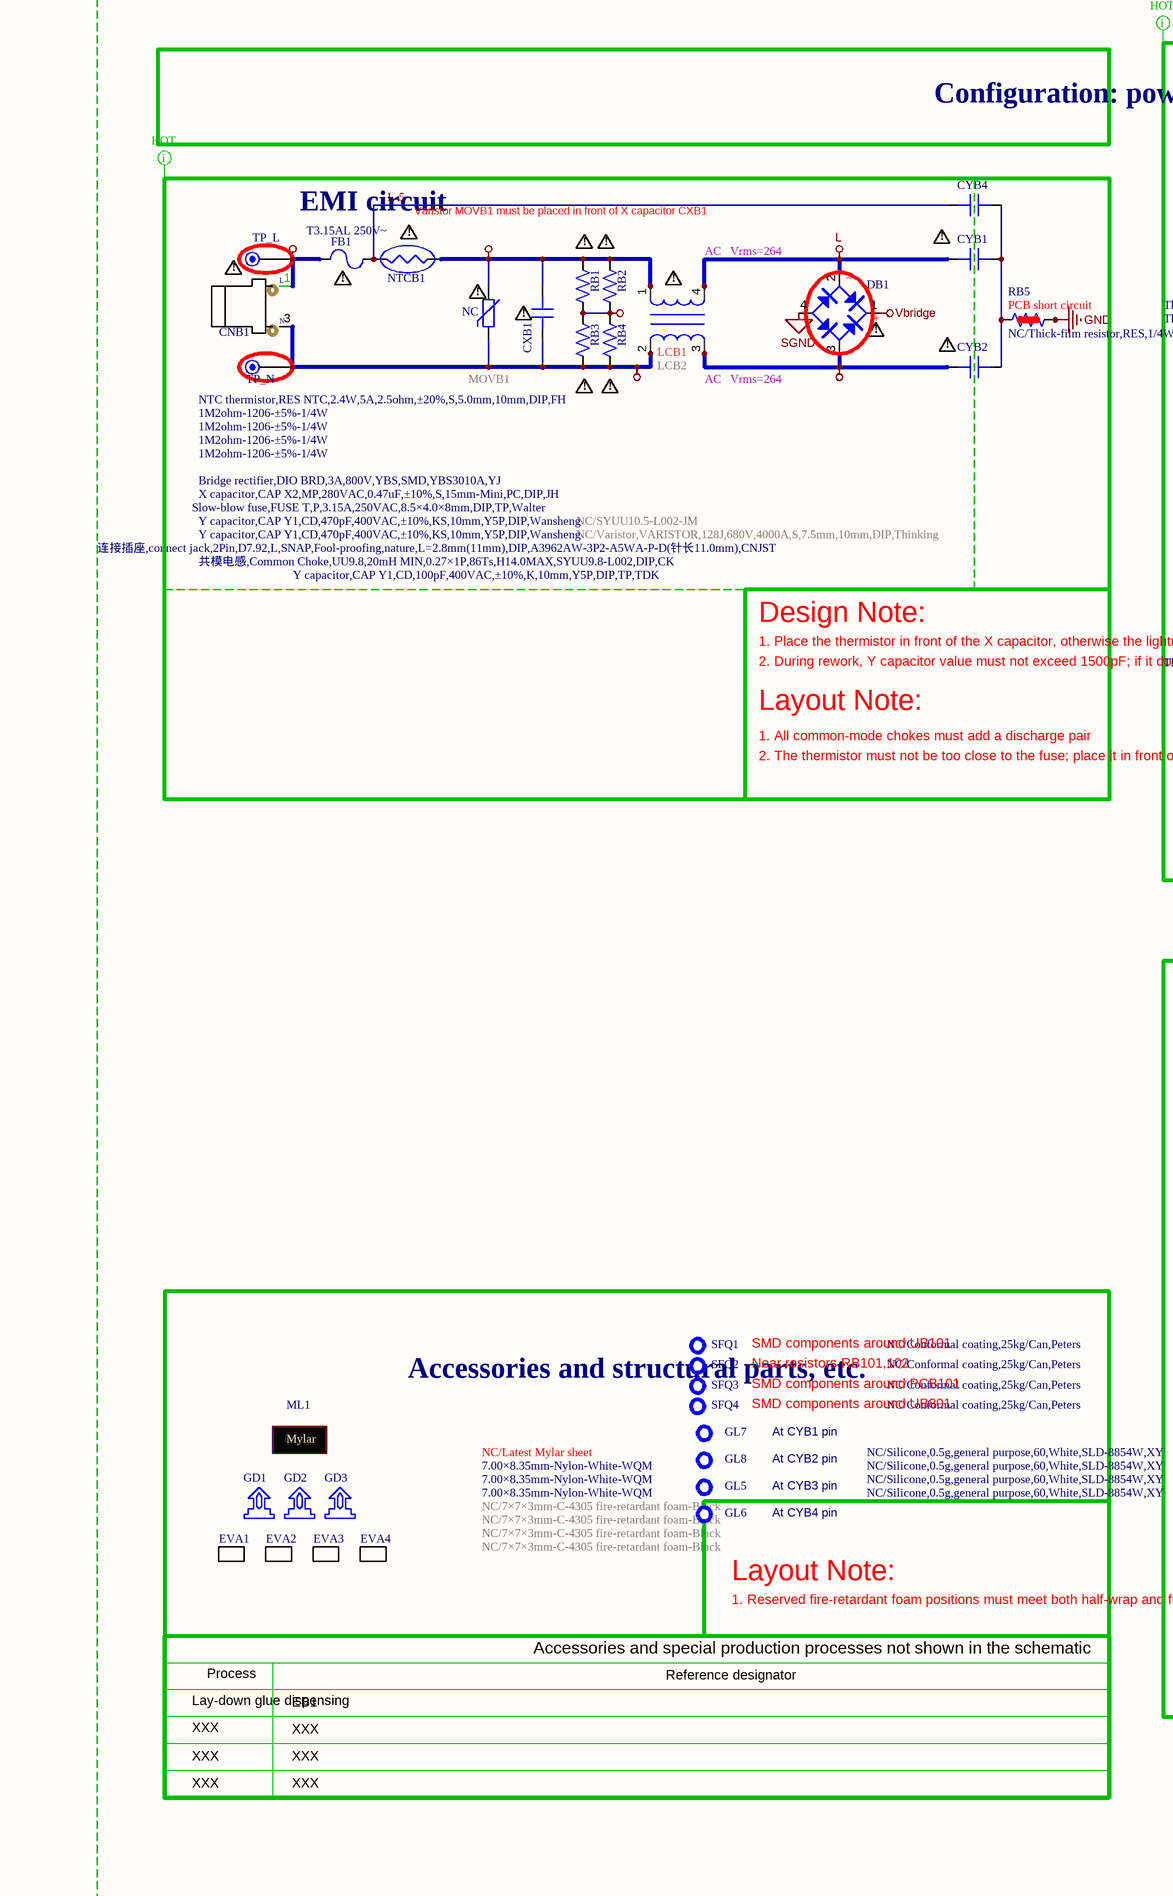
[diagram p0: MISC116569-4.SchDoc, left]
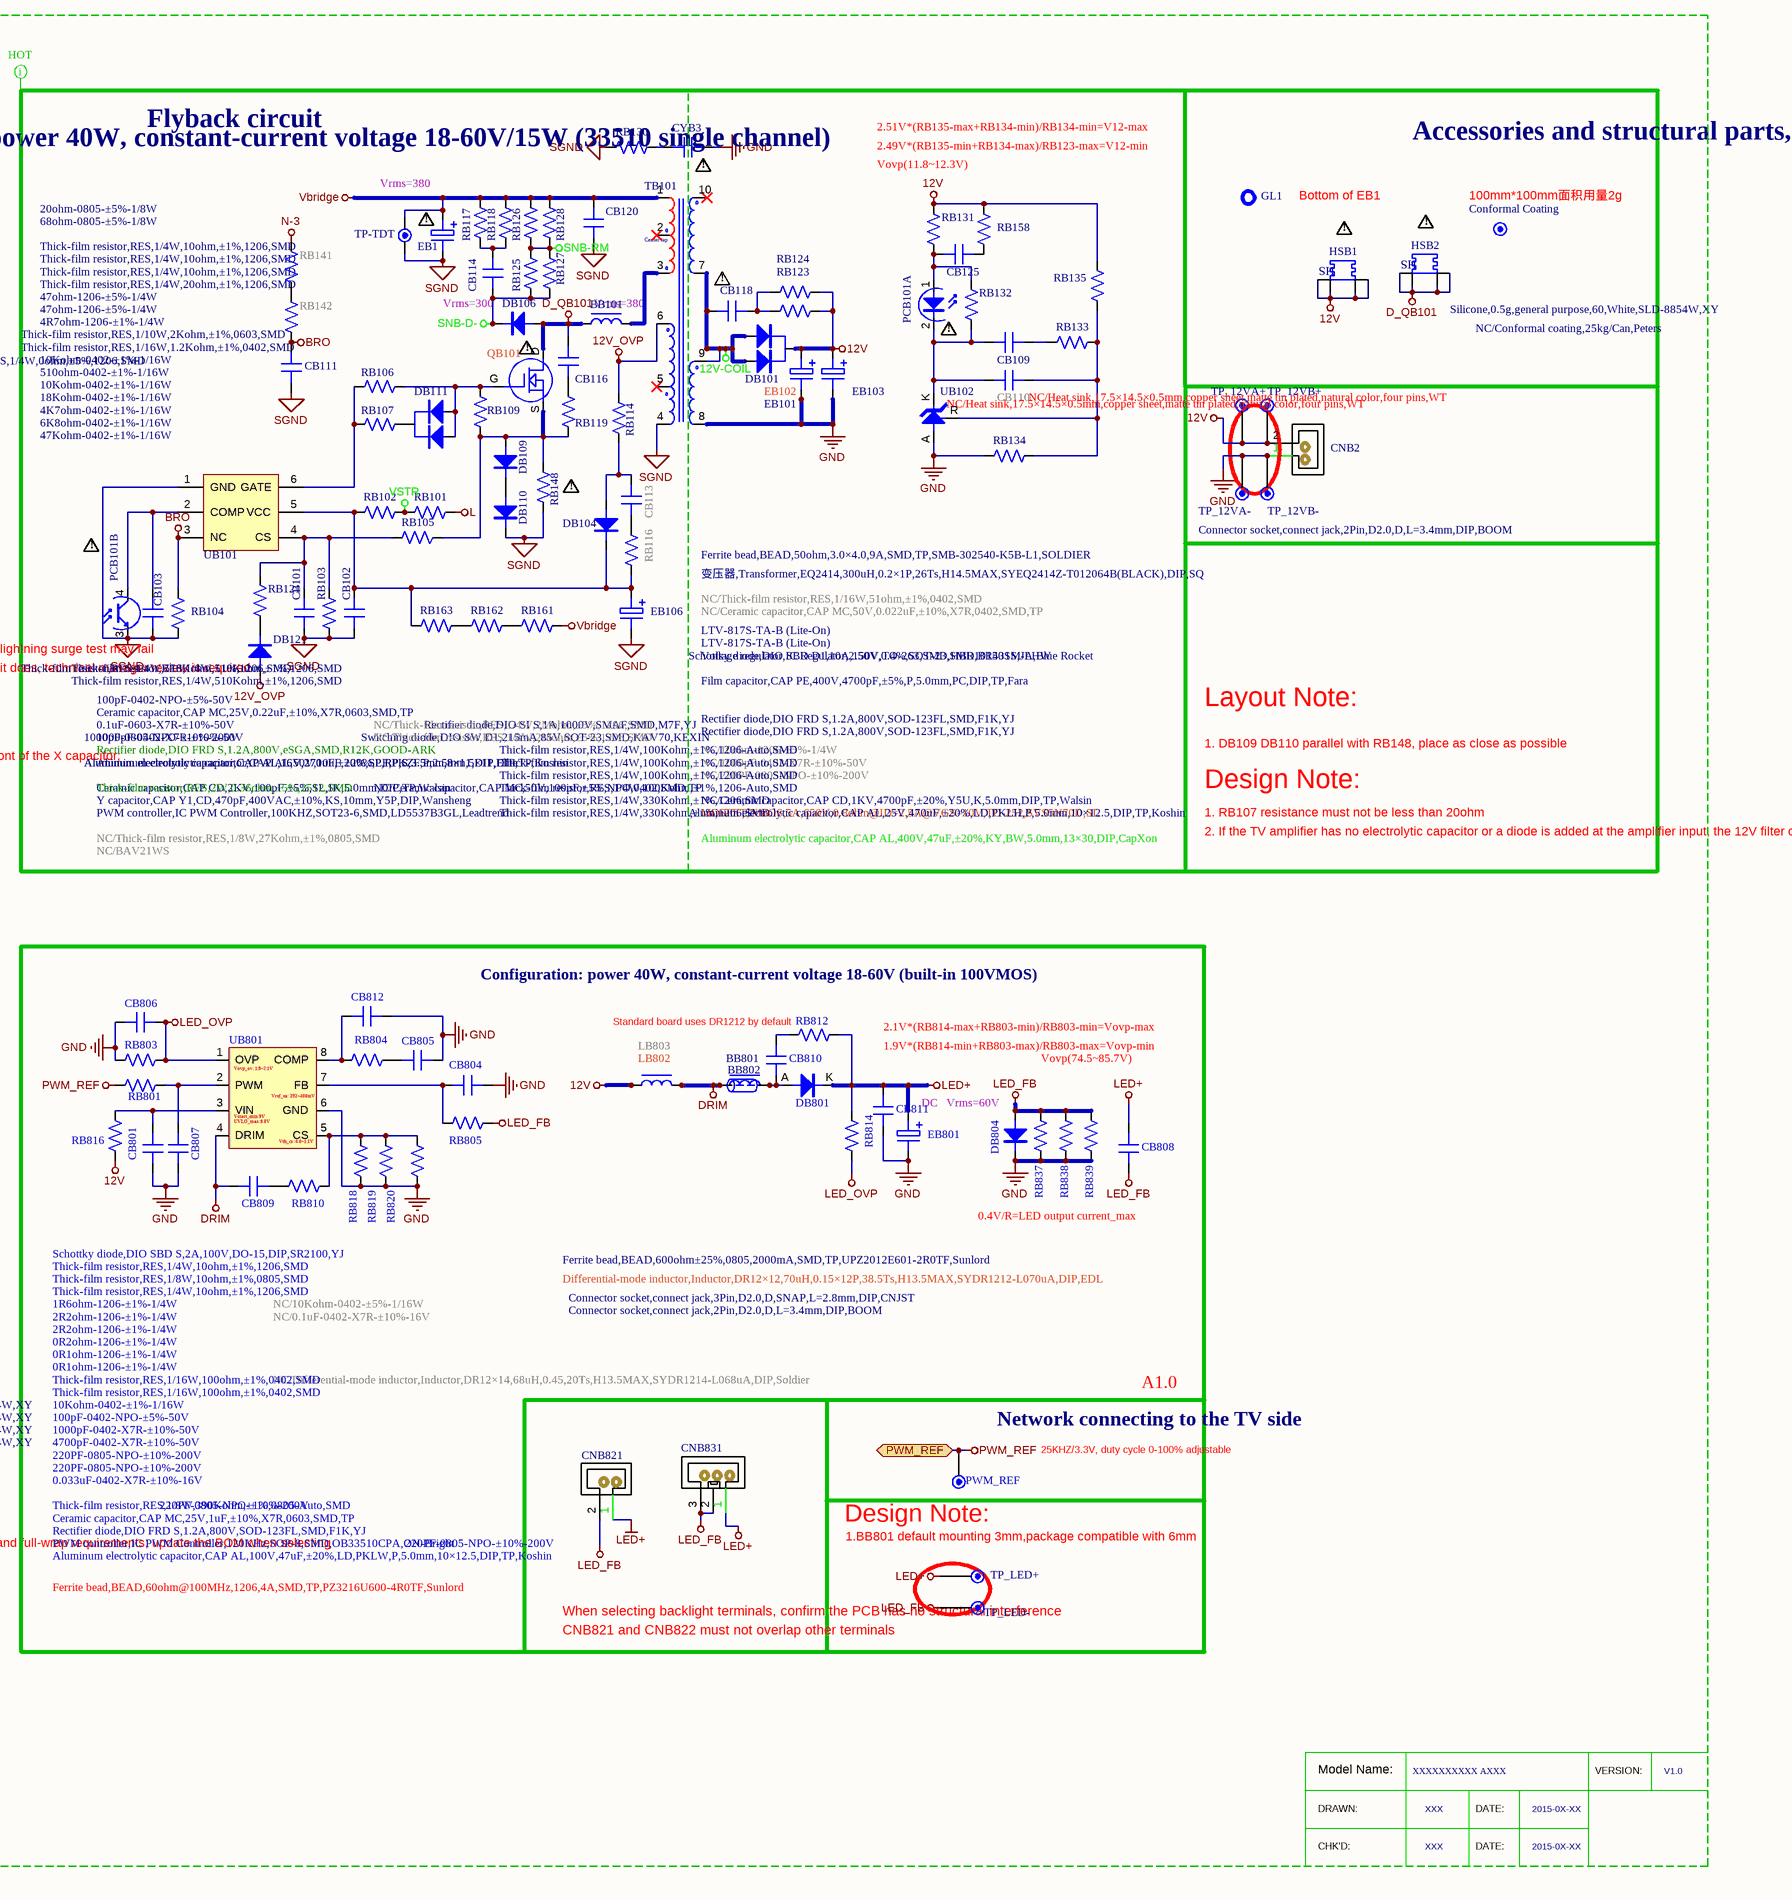
[diagram p1: MISC116569-4.SchDoc, right]
# Altium project MISC116569-15.PrjPCB (part 7 of 8)

## Sheet MISC116569-4.SchDoc: MISC116569
size A2

### Parts
BB101  Ferrite bead,BEAD,50ohm,3.0×4.0,9A,SMD,TP,SMB-302540-K5B-L1,SOLDIER  [L(4*3*2.55)-S]
BB801  Ferrite bead,BEAD,60ohm@100MHz,1206,4A,SMD,TP,PZ3216U600-4R0TF,Sunlord  [L1206]
BB802  Ferrite bead,BEAD,600ohm±25%,0805,2000mA,SMD,TP,UPZ2012E601-2R0TF,Sunlord  [L0805]
CB101  100pF-0402-NPO-±5%-50V  [C0402]
CB102  0.1uF-0603-X7R-±10%-50V  [C0603]
CB103  1000pF-0402-X7R-±10%-50V  [C0402]
CB109  Ceramic capacitor,CAP MC,25V,0.22uF,±10%,X7R,0603,SMD,TP  [C0603]
CB110  NC/1000pF-0402-X7R-±10%-50V  [C0402]
CB111  NC/Ceramic capacitor,CAP MC,50V,100pF,±5%,NPO,0402,SMD,TP  [C0402]
CB113  NC/220PF-0805-NPO-±10%-200V  [C0805]
CB114  Film capacitor,CAP PE,400V,4700pF,±5%,P,5.0mm,PC,DIP,TP,Fara  [CAP8*2.5-V-5]
CB116  Ceramic capacitor,CAP CD,2KV,100pF,±5%,SL,IK,5.0mm,DIP,TP,Walsin  [CAP6.5*5-V-5-1]
CB118  1000pF-0805-NPO-±10%-200V  [C0805]
CB120  NC/Ceramic capacitor,CAP CD,1KV,4700pF,±20%,Y5U,K,5.0mm,DIP,TP,Walsin  [CAP10*4.5-V-5]
CB125  NC/Ceramic capacitor,CAP MC,50V,0.022uF,±10%,X7R,0402,SMD,TP  [C0402]
CB801  Ceramic capacitor,CAP MC,25V,1uF,±10%,X7R,0603,SMD,TP  [C0603]
CB804  4700pF-0402-X7R-±10%-50V  [C0402]
CB805  NC/0.1uF-0402-X7R-±10%-16V  [C0402]
CB806  1000pF-0402-X7R-±10%-50V  [C0402]
CB807  100pF-0402-NPO-±5%-50V  [C0402]
CB808  220PF-0805-NPO-±10%-200V  [C0805]
CB809  220PF-0805-NPO-±10%-200V  [C0805]
CB810  220PF-0805-NPO-±10%-200V  [C0805]
CB811  220PF-0805-NPO-±10%-200V  [C0805]
CB812  0.033uF-0402-X7R-±10%-16V  [C0402]
CNB1  连接插座,connect jack,2Pin,D7.92,L,SNAP,Fool-proofing,nature,L=2.8mm(11mm),DIP,A3962AW-3P2-A5WA-P-D(针长11.0mm),CNJST  [CON2-H7.92]
CNB2  Connector socket,connect jack,2Pin,D2.0,D,L=3.4mm,DIP,BOOM  [SIP2/2.0D-1]
CNB821  Connector socket,connect jack,2Pin,D2.0,D,L=3.4mm,DIP,BOOM  [SIP2/2.0D-1]
CNB831  Connector socket,connect jack,3Pin,D2.0,D,SNAP,L=2.8mm,DIP,CNJST  [SIP3/2.0D-3]
Conformal_Coating  NC/Conformal coating,25kg/Can,Peters  [Conformal Coating]
CXB1  X capacitor,CAP X2,MP,280VAC,0.47uF,±10%,S,15mm-Mini,PC,DIP,JH  [CAP18*8.5-V-15]
CYB1  Y capacitor,CAP Y1,CD,470pF,400VAC,±10%,KS,10mm,Y5P,DIP,Wansheng  [CAP13*5-V-10-1]
CYB2  Y capacitor,CAP Y1,CD,470pF,400VAC,±10%,KS,10mm,Y5P,DIP,Wansheng  [CAP13*5-V-10-1]
CYB3  Y capacitor,CAP Y1,CD,470pF,400VAC,±10%,KS,10mm,Y5P,DIP,Wansheng  [CAP13*5-V-10-1]
CYB4  Y capacitor,CAP Y1,CD,100pF,400VAC,±10%,K,10mm,Y5P,DIP,TP,TDK  [CAP13*5-V-10-1]
DB1  Bridge rectifier,DIO BRD,3A,800V,YBS,SMD,YBS3010A,YJ  [B/YBS3010A]
DB101  Schottky diode,DIO SBD D1,10A,150V,TO-263,SMD,HBR10150SS,JLHW  [D2PAK3]
DB104  Rectifier diode,DIO SI S,1A,1000V,SMAF,SMD,M7F,YJ  [DIODE-S-1]
DB106  Rectifier diode,DIO FRD S,1.2A,800V,eSGA,SMD,R12K,GOOD-ARK  [DIODE-S-14]
DB109  Rectifier diode,DIO FRD S,1.2A,800V,SOD-123FL,SMD,F1K,YJ  [DIODE-S-14]
DB110  Rectifier diode,DIO FRD S,1.2A,800V,SOD-123FL,SMD,F1K,YJ  [DIODE-S-14]
DB111  Switching diode,DIO SW D1,215mA,85V,SOT-23,SMD,KAV70,KEXIN  [SO-23]
DB121  NC/BAV21WS  [DIODE-S-12]
DB801  Schottky diode,DIO SBD S,2A,100V,DO-15,DIP,SR2100,YJ  [D2-H-15]
DB804  Rectifier diode,DIO FRD S,1.2A,800V,SOD-123FL,SMD,F1K,YJ  [DIODE-S-14]
EB1  Aluminum electrolytic capacitor,CAP AL,400V,47uF,±20%,KY,BW,5.0mm,13×30,DIP,CapXon  [EC(13*30)-H-5]
EB101  Aluminum electrolytic capacitor,CAP AL,16V,270uF,±20%,SP,RP,S,3.5mm,8×11,DIP,Elite  [EC(8*11)-V-3.5]
EB102  Aluminum electrolytic capacitor,CAP AL,25V,470uF,±20%,LD,PKLH,P,5.0mm,10×12.5,DIP,TP,Koshin  [EC(10*12.5)-V-5]
EB103  Aluminum electrolytic capacitor,CAP AL,16V,270uF,±20%,SP,RP,S,3.5mm,8×11,DIP,Elite  [EC(8*11)-V-3.5]
EB106  Aluminum electrolytic capacitor,CAP AL,50V,10uF,±20%,LF,PKZF,P,2.5mm,5×11,DIP,TP,Koshin  [EC(5*11)-V-2.5]
EB801  Aluminum electrolytic capacitor,CAP AL,100V,47uF,±20%,LD,PKLW,P,5.0mm,10×12.5,DIP,TP,Koshin  [EC(10*12.5)-V-5]
EVA1  NC/7×7×3mm-C-4305 fire-retardant foam-Black  [EVA(7*7*3)]
EVA2  NC/7×7×3mm-C-4305 fire-retardant foam-Black  [EVA(7*7*3)]
EVA3  NC/7×7×3mm-C-4305 fire-retardant foam-Black  [EVA(7*7*3)]
EVA4  NC/7×7×3mm-C-4305 fire-retardant foam-Black  [EVA(7*7*3)]
FB1  Slow-blow fuse,FUSE T,P,3.15A,250VAC,8.5×4.0×8mm,DIP,TP,Walter  [FUSE8.5*4-V-5(T3.15AL 250V~)]
GD1  7.00×8.35mm-Nylon-White-WQM  [Fixed]
GD2  7.00×8.35mm-Nylon-White-WQM  [Fixed]
GD3  7.00×8.35mm-Nylon-White-WQM  [Fixed]
GL1  Silicone,0.5g,general purpose,60,White,SLD-8854W,XY  [Silica gel-15]
GL5  NC/Silicone,0.5g,general purpose,60,White,SLD-8854W,XY  [Silica gel-10]
GL6  NC/Silicone,0.5g,general purpose,60,White,SLD-8854W,XY  [Silica gel-10]
GL7  NC/Silicone,0.5g,general purpose,60,White,SLD-8854W,XY  [Silica gel-10]
GL8  NC/Silicone,0.5g,general purpose,60,White,SLD-8854W,XY  [Silica gel-10]
HSB1  NC/Heat sink,17.5×14.5×0.5mm,copper sheet,matte tin plated,natural color,four pins,WT  [HS151-TEMP-NG]
HSB2  NC/Heat sink,17.5×14.5×0.5mm,copper sheet,matte tin plated,natural color,four pins,WT  [HS151-TEMP-NG]
LB802  Differential-mode inductor,Inductor,DR12×12,70uH,0.15×12P,38.5Ts,H13.5MAX,SYDR1212-L070uA,DIP,EDL  [L/LC2/15*14.5-V7.5]
LB803  NC/Differential-mode inductor,Inductor,DR12×14,68uH,0.45,20Ts,H13.5MAX,SYDR1214-L068uA,DIP,Soldier  [L(13.5*15.5)-V-5]
LCB1  共模电感,Common Choke,UU9.8,20mH MIN,0.27×1P,86Ts,H14.0MAX,SYUU9.8-L002,DIP,CK  [L/LC4/UU9.8/7*8-H]
LCB2  NC/SYUU10.5-L002-JM  [L/UU10.5/10*13-2]
ML1  NC/Latest Mylar sheet  [Mylar]
MOVB1  NC/Varistor,VARISTOR,128J,680V,4000A,S,7.5mm,10mm,DIP,Thinking  [VR(13*5)-V-7.5]
NTCB1  NTC thermistor,RES NTC,2.4W,5A,2.5ohm,±20%,S,5.0mm,10mm,DIP,FH  [NTC(10*5)-V5]
PCB101  LTV-817S-TA-B (Lite-On)  [OC4-S-1]  (parts A,B of 2)
PWM_REF  NC/TEST  [TP_BL]  (value not drawn)
QB101  MOSFET,NMOS,5A,650V,0.8ohm@ID=2.5A@VGS=10V,TO-252,SVS5N70D,SL  [TO-252-GDS]
RB1  1M2ohm-1206-±5%-1/4W  [R1206]
RB2  1M2ohm-1206-±5%-1/4W  [R1206]
RB3  1M2ohm-1206-±5%-1/4W  [R1206]
RB4  1M2ohm-1206-±5%-1/4W  [R1206]
RB5  NC/Thick-film resistor,RES,1/4W,0ohm,±5%,1206,SMD  [R1206SC]
RB101  Thick-film resistor,RES,1/4W,330Kohm,±1%,1206,SMD  [R1206]
RB102  Thick-film resistor,RES,1/4W,330Kohm,±1%,1206,SMD  [R1206]
RB103  6K8ohm-0402-±1%-1/16W  [R0402]
RB104  47Kohm-0402-±1%-1/16W  [R0402]
RB105  510ohm-0402-±1%-1/16W  [R0402]
RB106  68ohm-0805-±5%-1/8W  [R0805]
RB107  20ohm-0805-±5%-1/8W  [R0805]
RB109  10Kohm-0402-±1%-1/16W  [R0402]
RB114  4R7ohm-1206-±1%-1/4W  [R1206]
RB116  NC/10ohm-1206-±5%-1/4W  [R1206]
RB117  Thick-film resistor,RES,1/4W,10ohm,±1%,1206,SMD  [R1206]
RB118  Thick-film resistor,RES,1/4W,10ohm,±1%,1206,SMD  [R1206]
RB119  Thick-film resistor,RES,1/4W,10ohm,±1%,1206,SMD  [R1206]
RB121  NC/Thick-film resistor,RES,1/8W,27Kohm,±1%,0805,SMD  [R0805]
RB123  47ohm-1206-±5%-1/4W  [R1206]
RB124  47ohm-1206-±5%-1/4W  [R1206]
RB125  Thick-film resistor,RES,1/4W,100Kohm,±1%,1206-Auto,SMD  [R1206]
RB126  Thick-film resistor,RES,1/4W,100Kohm,±1%,1206-Auto,SMD  [R1206]
RB127  Thick-film resistor,RES,1/4W,100Kohm,±1%,1206-Auto,SMD  [R1206]
RB128  Thick-film resistor,RES,1/4W,100Kohm,±1%,1206-Auto,SMD  [R1206]
RB130  Thick-film resistor,RES,1/4W,20ohm,±1%,1206,SMD  [R1206]
RB131  Thick-film resistor,RES,1/10W,2Kohm,±1%,0603,SMD  [R0603]
RB132  Thick-film resistor,RES,1/16W,1.2Kohm,±1%,0402,SMD  [R0402]
RB133  10Kohm-0402-±1%-1/16W  [R0402]
RB134  4K7ohm-0402-±1%-1/16W  [R0402]
RB135  18Kohm-0402-±1%-1/16W  [R0402]
RB141  NC/Thick-film resistor,RES,1/4W,2Mohm,±5%,1206,SMD  [R1206]
RB142  NC/Thick-film resistor,RES,1/4W,2Mohm,±5%,1206,SMD  [R1206]
RB148  Thick-film resistor,RES,2W,0.36ohm,±5%,2512,SMD  [R2512-1]
RB158  NC/Thick-film resistor,RES,1/16W,51ohm,±1%,0402,SMD  [R0402]
RB161  Thick-film resistor,RES,1/4W,510Kohm,±1%,1206,SMD  [R1206]
RB162  Thick-film resistor,RES,1/4W,510Kohm,±1%,1206,SMD  [R1206]
RB163  Thick-film resistor,RES,1/4W,510Kohm,±1%,1206,SMD  [R1206]
RB801  Thick-film resistor,RES,1/16W,100ohm,±1%,0402,SMD  [R0402]
RB803  10Kohm-0402-±1%-1/16W  [R0402]
RB804  NC/10Kohm-0402-±5%-1/16W  [R0402]
RB805  Thick-film resistor,RES,1/16W,100ohm,±1%,0402,SMD  [R0402]
RB810  Thick-film resistor,RES,1/4W,10ohm,±1%,1206,SMD  [R1206]
RB812  Thick-film resistor,RES,1/4W,10ohm,±1%,1206,SMD  [R1206]
RB814  Thick-film resistor,RES,1/8W,390Kohm,±1%,0805-Auto,SMD  [R0805]
RB816  Thick-film resistor,RES,1/8W,10ohm,±1%,0805,SMD  [R0805]
RB818  0R2ohm-1206-±1%-1/4W  [R1206]
RB819  0R1ohm-1206-±1%-1/4W  [R1206]
RB820  0R1ohm-1206-±1%-1/4W  [R1206]
RB837  1R6ohm-1206-±1%-1/4W  [R1206]
RB838  2R2ohm-1206-±1%-1/4W  [R1206]
RB839  2R2ohm-1206-±1%-1/4W  [R1206]
SFQ1  NC/Conformal coating,25kg/Can,Peters  [SFQ]
SFQ2  NC/Conformal coating,25kg/Can,Peters  [SFQ]
SFQ3  NC/Conformal coating,25kg/Can,Peters  [SFQ]
SFQ4  NC/Conformal coating,25kg/Can,Peters  [SFQ]
TB101  变压器,Transformer,EQ2414,300uH,0.2×1P,26Ts,H14.5MAX,SYEQ2414Z-T012064B(BLACK),DIP,SQ  [T/EQ2414*10]
TP-TDT  NC/  [TP-TDT]  (value not drawn)
TP_12VA+  NC/  [TP]  (value not drawn)
TP_12VA-  NC/  [TP]  (value not drawn)
TP_12VB+  NC/  [TP]  (value not drawn)
TP_12VB-  NC/  [TP]  (value not drawn)
TP_L  NC/  [TP-80]  (value not drawn)
TP_LED+  NC/  [TP]  (value not drawn)
TP_LED-  NC/  [TP]  (value not drawn)
TP_N  NC/  [TP-80]  (value not drawn)
UB101  PWM controller,IC PWM Controller,100KHZ,SOT23-6,SMD,LD5537B3GL,Leadtrend  [SOT-26]
UB102  Voltage regulator,IC Regulator,2.50V,0.4%,SOT-23,SMD,BR431M-A,Blue Rocket  [SOT-23-RAK]
UB801  PWM controller,IC PWM Controller,120KHz,SOP-8,SMD,OB33510CPA,ON-Bright  [SO-8A]

### Blocks framed on the sheet
Design Note:: BB801 BB802 CB801 CB804-CB812 CNB821 CNB831 DB801 DB804 EB801 LB802 LB803 PWM_REF RB801 RB803-RB805 RB810 RB812 RB814 RB816 RB818-RB820 RB837-RB839 TP_LED+ TP_LED- UB801

### Ports
PWM_REF

### Nets
12V: CNB2.2 DB101.2 EB101.1 EB102.1 EB103.1 HSB1.1 HSB1.2 HSB1.3 HSB1.4 LB802.1 LB803.1 RB123.2 RB124.2 RB131.2 RB135.1 RB158.2 RB816.1 TP_12VA+.1 TP_12VB+.1
12V-COIL: CB118.1 DB101.1 DB101.3 TB101.7 TB101.9
12V_OVP: DB121.A RB114.2 TB101.6
BRO: CB111.1 RB104.1 RB142.1 UB101.3(NC)
D_QB101: BB101.1 CB116.2 DB106.A HSB2.1 HSB2.2 HSB2.3 HSB2.4 QB101.D
DRIM: BB801.1 BB802.1 CB809.2 LB802.2 LB803.2 UB801.4(DRIM)
GND: CB801.2 CB804.1 CB805.2 CB806.2 CB807.1 CB811.1 CB812.2 CNB2.1 CYB3.2 DB804.K EB101.2 EB102.2 EB103.2 EB801.2 RB5.2 RB5.3 RB134.1 RB803.1 RB818.1 RB819.1 RB820.1 RB837.1 RB838.1 RB839.2 TB101.8 TP_12VA-.1 TP_12VB-.1 UB102.A UB801.6(GND)
L: CYB1.1 DB1.2 LCB1.4 LCB2.4 RB101.1
L-1: CNB1.1 FB1.1 TP_L.1
L-2: CXB1.1 LCB1.1 LCB2.1 MOVB1.1 NTCB1.1 RB1.1 RB2.1
L-N: RB1.2 RB2.2 RB3.1 RB4.1
LED+: CB808.2 CB811.2 CNB821.1 CNB831.1 DB801.K EB801.1 RB812.2 RB814.2 TP_LED+.1
LED_FB: CB808.1 CNB821.2 CNB831.2 CNB831.3 DB804.A RB805.2 RB837.2 RB838.2 RB839.1 TP_LED-.1
LED_OVP: CB806.1 RB803.2 RB814.1 UB801.1(OVP)
N-2: CNB1.3 CXB1.2 LCB1.2 LCB2.2 MOVB1.2 RB3.2 RB4.2 TP_N.1
N-3: CYB2.1 DB1.3 LCB1.3 LCB2.3 RB141.2
PWM_REF: PWM_REF.1 RB801.1 ; port PWM_REF
SGND: CB101.2 CB102.2 CB103.1 CB111.2 CB120.1 DB1.4 DB110.K EB1.2 EB106.2 PCB101.3 RB103.1 RB104.2 RB130.1 RB148.1 TB101.4 TP-TDT.2 UB101.1(GND)
SNB-D-: CB114.2 DB106.K RB125.1 RB127.1
SNB-RM: RB125.2 RB126.1 RB127.2 RB128.1
Vbridge: CB120.2 DB1.1 EB1.1 RB117.2 RB118.2 RB126.2 RB128.2 RB161.1 TB101.1 TP-TDT.1
VSTR: RB101.2 RB102.1
L-5: CYB4.1 FB1.2 NTCB1.2
NetBB101_2: BB101.2 TB101.3
NetBB801_2: BB801.2 BB802.2 CB810.1 DB801.A
NetCB101_1: CB101.1 RB103.2 RB105.1 RB121.2 UB101.4(CS)
NetCB102_1: CB102.1 DB104.K EB106.1 RB102.2 RB116.1 RB163.2 UB101.5(VCC)
NetCB103_2: CB103.2 PCB101.4 UB101.2(COMP)
NetCB109_1: CB109.1 CB110.1 PCB101.2 RB132.1 UB102.K
NetCB109_2: CB109.2 RB133.1
NetCB110_2: CB110.2 RB133.2 RB134.2 RB135.2 UB102.R
NetCB113_1: CB113.1 DB104.A RB114.1
NetCB113_2: CB113.2 RB116.2
NetCB114_1: CB114.1 RB117.1 RB118.1
NetCB116_1: CB116.1 RB119.2
NetCB118_2: CB118.2 RB123.1 RB124.1
NetCB125_1: CB125.1 PCB101.1 RB131.1 RB132.2
NetCB125_2: CB125.2 RB158.1
NetCB801_1: CB801.1 RB816.2 UB801.3(VIN)
NetCB804_2: CB804.2 RB805.1 UB801.7(FB)
NetCB805_1: CB805.1 RB804.2
NetCB807_2: CB807.2 RB801.2 UB801.2(PWM)
NetCB809_1: CB809.1 RB810.2
NetCB810_2: CB810.2 RB812.1
NetCB812_1: CB812.1 RB804.1 UB801.8(COMP)
NetCYB1_2: CYB1.2 CYB2.2 CYB4.2 RB5.1
NetCYB3_1: CYB3.1 RB130.2
NetDB109_A: DB109.A QB101.S RB105.2 RB109.2 RB119.1 RB148.2
NetDB109_K: DB109.K DB110.A
NetDB111_1: DB111.1 DB111.3 QB101.G RB106.2 RB109.1
NetDB111_2: DB111.2 RB107.2
NetDB121_K: DB121.K RB121.1
NetRB106_1: RB106.1 RB107.1 UB101.6(GATE)
NetRB141_1: RB141.1 RB142.2
NetRB161_2: RB161.2 RB162.1
NetRB162_2: RB162.2 RB163.1
NetRB810_1: RB810.1 RB818.2 RB819.2 RB820.2 UB801.5(CS)

Not connected (* = marked no-connect by the designer): TB101 2* 5* 10*

### Layout directives
net class HOT: 12V_OVP, BRO, D_QB101, L, L-1, L-2, L-5, L-N, N-2, N-3, SGND, SNB-D-, SNB-RM, Vbridge, VSTR
net class POWER: 12V, 12V-COIL, 12V_OVP, BRO, D_QB101, DRIM, GND, L, L-1, L-2, L-5, L-N, LED+, LED_FB, LED_OVP, N-2, N-3, PWM_REF, SGND, SNB-D-, SNB-RM, Vbridge, VSTR

### Notes on the sheet
- Configuration: power 40W, constant-current voltage 18-60V/15W (33510 single channel)
- Flyback circuit
- Vrms=380
- (near CYB3) !
- 2.51V*(RB135-max+RB134-min)/RB134-min=V12-max
- 2.49V*(RB135-min+RB134-max)/RB123-max=V12-min
- Vovp(11.8~12.3V)
- Accessories and structural parts, etc.
- EMI circuit
- Varistor MOVB1 must be placed in front of X capacitor CXB1
- !
- Bottom of EB1
- (near HSB1) !
- (near HSB2) !
- (near Conformal_Coating) 100mm*100mm面积用量2g
- (near FB1) !
- (near NTCB1) !
- AC   Vrms=264
- Vrms=300
- (near BB101) Vrms=380
- (near MOVB1) NC
- (near MOVB1) !
- (near CXB1) !
- (near DB1) !
- (near CYB2) !
- (near QB101) !
- 1. Place the thermistor in front of the X capacitor, otherwise the lightning surge test may fail
- (near DB121) 2. During rework, Y capacitor value must not exceed 1500pF; if it does, technical manager review is required
- Design Note:
- Layout Note:
- 1. All common-mode chokes must add a discharge pair
- 1. DB109 DB110 parallel with RB148, place as close as possible
- 2. The thermistor must not be too close to the fuse; place it in front of the X capacitor;
- 1. RB107 resistance must not be less than 20ohm
- 2. If the TV amplifier has no electrolytic capacitor or a diode is added at the amplifier input, the 12V filter cannot use solid-state capacitors; two aluminum electrolytic capacitors are required
- Configuration: power 40W, constant-current voltage 18-60V (built-in 100VMOS)
- (near RB812) Standard board uses DR1212 by default
- 2.1V*(RB814-max+RB803-min)/RB803-min=Vovp-max
- 1.9V*(RB814-min+RB803-max)/RB803-max=Vovp-min
- Vovp(74.5~85.7V)
- DC   Vrms=60V
- 0.4V/R=LED output current_max
- SMD components around UB101
- Near resistors RB101,102
- (near ML1) Accessories and structural parts, etc.
- SMD components around PCB101
- SMD components around UB801
- At CYB2 pin
- At CYB3 pin
- At CYB1 pin
- Network connecting to the TV side
- 25KHZ/3.3V, duty cycle 0-100% adjustable
- A1.0
- At CYB4 pin
- 1. Reserved fire-retardant foam positions must meet both half-wrap and full-wrap requirements; update the BOM when selecting
- (near TP_LED+) 1.BB801 default mounting 3mm,package compatible with 6mm
- Process
- Accessories and special production processes not shown in the schematic
- Reference designator
- CNB821 and CNB822 must not overlap other terminals
- (near TP_LED-) When selecting backlight terminals, confirm the PCB has no structural interference
- Lay-down glue dispensing
- XXX
- EB1
- Model Name:
- DRAWN:
- XXXXXXXXXX AXXX
- DATE:
- 2015-0X-XX
- VERSION:
- V1.0
- CHK'D:
- Title
- Size:
- Date:
- A4
- Number:
- Time:
- Revision:
- Sheet
- of
- File:

### Library data of the parts
BB101 = 004.004.0001046-D: Ferrite bead,BEAD,50ohm,3.0×4.0,9A,SMD,TP,SMB-302540-K5B-L1,SOLDIER-D
BB801 = UPZ2012E601-2R0TF(600ohm-2000mA)
BB802 = 004.004.0000340-D: Ferrite bead,BEAD,600ohm±25%,0805,2000mA,SMD,TP,UPZ2012E601-2R0TF,Sunlord-D
CB101 CB111 CB807 = 100pF-0402-NPO-±5%-50V-D
CB102 CB109 = 0.1uF-0603-X7R-±10%-50V-D: CAP
CB103 CB806 = 1000pF-0402-X7R-±10%-50V-D
CB110 CB125 = 1000pF-0402-X7R-±10%-50V-D: CAP
CB113 CB808-CB811 = 220PF-0805-NPO-±10%-200V-D: CAP
CB114 = C242G472J20A201(编带/法拉)-DAI: CAP
CB116 = 004.003.0001889-DHAI: Ceramic capacitor,CAP CD,1KV,100pF,±5%,SL,OK,5.0mm,DIP,TP,TDK-DHAI
CB118 = 1000pF-0805-NPO-±10%-200V-D: CAP
CB120 = 004.003.0001665: Ceramic capacitor,CAP CD,1KV,4700pF,±20%,Y5U,K,5.0mm,DIP,TP,Walsin-DHAI
CB801 = 1uf-0603-X7R-±10%-25V-D
CB804 = 4700pF-0402-X7R-±10%-50V-D
CB805 = 0.1uF-0402-X7R-±10%-16V-D
CB812 = 0.033uF-0402-X7R-±10%-16V-D
CNB1 = 连接插座,connect jack,2Pin,D7.92,L,SNAP,Fool-proofing,nature,L=2.8mm,DIP,AMA-DLMI: AC socket
CNB2 = XXX.XXX.0001753: Connector socket,connect jack,2Pin,D2.0,D,L=2.8mm,DIP,AMA-DHMI
CNB821 = XXX.XXX.0000603-DHMI: Connector socket,connect jack,2Pin,D2.0,D,L=3.4mm,DIP,BOOM-DHMI
CNB831 = XXX.XXX.0000643-DHMI: Connector socket,connect jack,3Pin,D2.0,D,SNAP,L=2.8mm,DIP,CNJST-DHMI
Conformal_Coating = 三防漆,25kg/Can,Peters
CXB1 = X电容,CAP X2,MP,275VAC,0.47uF,±10%,S,15mm-Mini,PC,DIP,BM-DHMI: CAP
CYB1-CYB4 = Y电容,CAP Y1,CD,470pF,400VAC,±20%,KS,10mm,Y5U,DIP,Walsin-DHMI: Y1 capacitor
DB1 = 004.005.0000860-D: Bridge rectifier,DIO BRD,3A,800V,YBS,SMD,YBS3010A,YJ-D
DB101 = MBRB10150CT(GOOD-ARK)-D: Diode
DB104 = M7(GOOD-ARK)-D
DB106 DB109 DB110 DB804 = 整流二极管,DIO FRD S,1.2A,800V,eSGA,SMD,R12K,GOOD-ARK-D
DB111 = LBAV70LT1G(LRC)-D: Diode
DB121 = BAV21WS-D: Diode
DB801 = SR210(编带/台半)-DLAI: Diode
EB1 = 47uF-400V-±20%-13×30-105℃-KY-折脚(H=11mm)(Capxon)-DLMI: Electrolytic
EB101 EB103 = 270uF-16V-±20%-8×11.5-105℃-PS-短脚-F=3.5(Capxon): Solid-state
EB102 = 470uF-25V-±20%-10×12.5-105℃-GF-编带-F=5.0(CapXon)-DHAI: Electrolytic
EB106 = 10uF-50V-±20%-5×11-105℃-GH-编带-F=2.5(CapXon)-DHAI: Electrolytic
EB801 = 47uF-100V-±20%-10×12-105℃-EV-编带-F=5.0(Elite)-DHAI: Electrolytic
EVA1-EVA4 = 7×7×3mm-C-4305防火泡棉-黑色-DLMI: EVA
FB1 = 004.026.0000010-DHMI: Slow-blow fuse,FUSE T,P,3.15A,250VAC,8.5×4.0×8mm,DIP,TP,Walter-DHMI
GD1-GD3 = 7.00×8.35mm-尼龙-白色-WQM-DHMI: Mylar stud
GL1 GL5-GL8 = 005.002.0000011: Silicone,0.2g,general purpose,60,White,SLD-8854W,XY-DHMI
HSB1 HSB2 = 004.040.0006600-DHMI: Heat sink,17.5×14.5×0.5mm,copper sheet,matte tin plated,natural color,four pins,WT-DHMI
LB802 = SYDR1212-L003-HM-DHMI: I-core inductor
LB803 = 差模电感,Inductor,DR12×14,68uH,0.45,20Ts,H13.5MAX,SYDR1214-L068uA,DIP,Soldier-DHMI: I-core inductor
LCB1 = SYUU9.8-L002-JM-DLMI: Common mode
LCB2 = SYUU10.5-L002-JM-DHMI: Common mode
ML1 = MALAY
MOVB1 = TVR10561KSW(为勤)-DHMI: Varistor
NTCB1 = SCK102R55AMBY502(短脚/为勤)-DHMI: Thermistor
PCB101 = LTV-817S-TA-B(光宝)-DMI: Optocoupler
PWM_REF TP-TDT TP_12VA+ TP_12VA- TP_12VB+ TP_12VB- TP_L TP_LED+ TP_LED- TP_N = TEST
QB101 = 场效应管,NMOS,5.2,650V,1.02ohm@ID=2.6A@VGS=10V,DPAK,TK5P65W,TOSHIBA-D: N Channel Single MOSFET
RB1-RB4 = 1M2ohm-1206-±5%-1/4W-D: RES
RB5 = 0ohm-1206-PCB-D
RB101 RB102 RB161-RB163 = 330Kohm-1206-±5%-1/4W-D: RES
RB103 = 6K8ohm-0402-±1%-1/16W-D
RB104 = 47Kohm-0402-±1%-1/16W-D
RB105 = 510ohm-0402-±1%-1/16W-D
RB106 RB121 = 68ohm-0805-±5%-1/8W-D
RB107 = 20ohm-0805-±5%-1/8W-D: RES
RB109 RB133 RB803 = 10Kohm-0402-±1%-1/16W-D
RB114 = 4R7ohm-1206-±1%-1/4W-D: RES
RB116-RB119 RB810 RB812 = 10ohm-1206-±5%-1/4W-D: RES
RB123 RB124 = 47ohm-1206-±5%-1/4W-D: RES
RB125-RB128 = 100Kohm-1206-±5%-1/4W-D: RES
RB130 = 20ohm-1206-±5%-1/4W-D
RB131 = 1Kohm-0603-±1%-1/10W-D
RB132 = 1Kohm-0402-±1%-1/16W-D
RB134 = 4K7ohm-0402-±1%-1/16W-D: RES
RB135 = 18Kohm-0402-±1%-1/16W-D: RES
RB141 RB142 = 2Mohm-1206-±5%-1/4W-D: RES
RB148 = 厚膜电阻,RES,1W,0.24ohm,±1%,2512,SMD
RB158 = 3Kohm-0402-±1%-1/16W-D
RB801 RB805 = 100ohm-0402-±5%-1/16W-D
RB804 = 10Kohm-0402-±5%-1/16W-D
RB814 = 390Kohm-0805-±1%-1/8W-D: RES
RB816 = 33ohm-0805-±5%-1/8W-D
RB818 = 0R2ohm-1206-±1%-1/4W-D
RB819 RB820 = 0R1ohm-1206-±1%-1/4W-D
RB837 = 1R6ohm-1206-±1%-1/4W-D: RES
RB838 RB839 = 2R2ohm-1206-±1%-1/4W-D: RES
SFQ1-SFQ4 = SFQ-D: NC/Conformal coating,25kg/Can,Peters-D
TB101 = 004.004.0002645-DLMI: 变压器,Transformer,EQ2414,300uH,0.2×1P,26Ts,H14.5MAX,SYEQ2414Z-T012064B(BLACK),DIP,SQ-DLMI
UB101 = PWM控制器,IC PWM Controller,65KHZ,SOT23-6,SMD,OB2273C,ON-Bright-D: IC
UB102 = AZ431AN-ATRE1(BCD)-D: SMD 431
UB801 = PWM控制器,IC PWM Controller,120KHz,SOP-8,SMD,OB3353LCPA,ON-Bright-D: IC